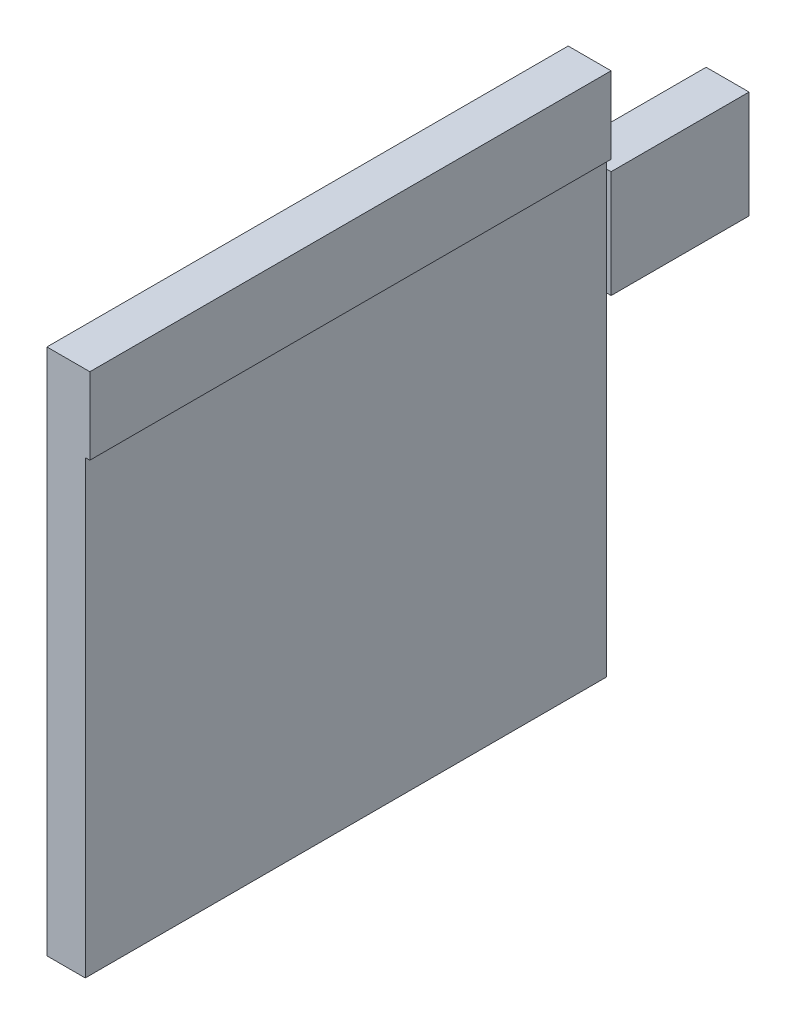
SolidWorks part; units mm, degrees
ref_plane "前视基准面" through (0, 0, 0) normal (0, 0, 1) x (1, 0, 0)
ref_plane "上视基准面" through (0, 0, 0) normal (0, 1, 0) x (1, 0, 0)
ref_plane "右视基准面" through (0, 0, 0) normal (1, 0, 0) x (0, 0, -1)
sketch "草图1" plane through (0, 0, 0) normal (0, 0, 1) x (1, 0, 0)
  line L0 (0, 0) -> (0, 172)
  line L1 (0, 172) -> (14, 172)
  line L2 (14, 172) -> (14, 147)
  line L3 (14, 147) -> (12.5, 147)
  line L4 (12.5, 147) -> (12.5, 0)
  line L5 (12.5, 0) -> (0, 0)
  dimension "D1" = 147
  dimension "D2" = 14
  dimension "D3" = 25
  dimension "D4" = 1.5
extrude "凸台-拉伸1" add sketch "草图1" along normal mid plane 170
sketch "草图2" plane through (0, 0, 0) normal (-1, 0, 0) x (0, 0, 1)
  line L0 (85, 0) -> (-85, 0) construction
  line L1 (-85, 172) -> (-85, 0) construction
  circle A0 centre (-73, 13) radius 6
  dimension "D1" = 12
  dimension "D2" = 13
  dimension "D3" = 12
extrude "切除-拉伸1" [suppressed] cut sketch "草图2" against normal blind 7
hole_wizard "M10x1.25 螺纹孔1" positions "3D草图1" profile "草图3" tap size "M10x1.25" standard "GB"
sketch3d "3D草图1" [suppressed]
  circle A0 centre (0, 13, -73) radius 6 construction
  point P0 (7, 13, -73)
  point P5 (-6, 13, -73)
sketch "草图3" plane through (7, 13, -73) normal (0, 1, 0) x (0, 0, 1)
  line L0 (0, 0) -> (0, 5.5)
  line L1 (0, 5.5) -> (4.4, 5.5)
  line L2 (4.4, 5.5) -> (4.4, 0)
  line L5 (4.4, 0) -> (0, 0)
  line L11 (0, -6.35) -> (0, 107.95) construction
  dimension "通孔螺纹孔钻头直径" = 8.8
  dimension "通孔螺纹孔钻头深度" = 5.5
cosmetic thread "孔螺蚊线1" parameters "D2"=10
sketch "草图4" plane through (0, 0, -85) normal (0, 0, -1) x (-1, 0, 0)
  line L0 (-14, 147) -> (-14, 172) construction
  line L1 (-14, 143.5) -> (0, 143.5)
  line L2 (-14, 143.5) -> (-14, 108.5)
  line L3 (-14, 108.5) -> (0, 108.5)
  line L4 (0, 143.5) -> (0, 108.5)
  line L5 (0, 172) -> (0, 0) construction
  line L6 (-14, 172) -> (0, 172) construction
  dimension "D1" = 28.5
  dimension "D2" = 35
extrude "凸台-拉伸2" add sketch "草图4" along normal blind 45
